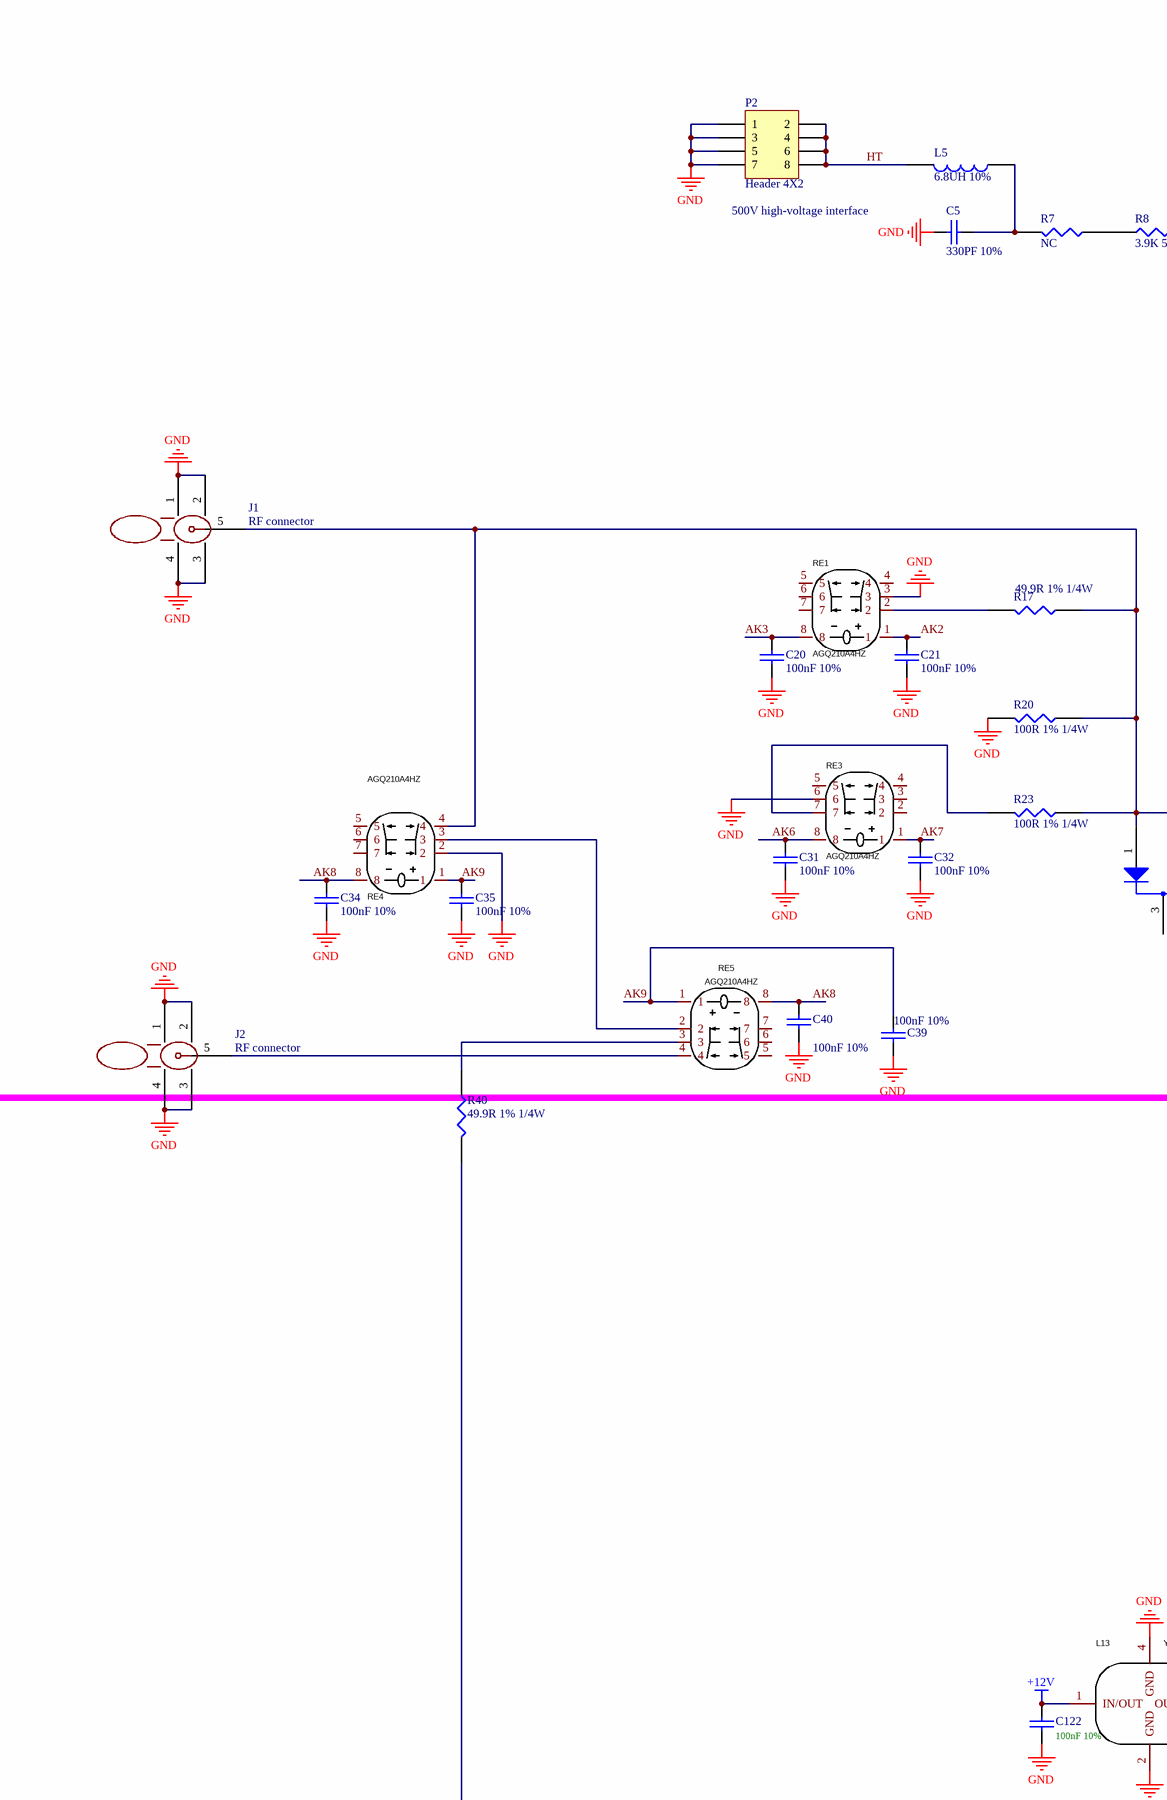
[diagram p0: PCBE109560-11.SchDoc, top left]
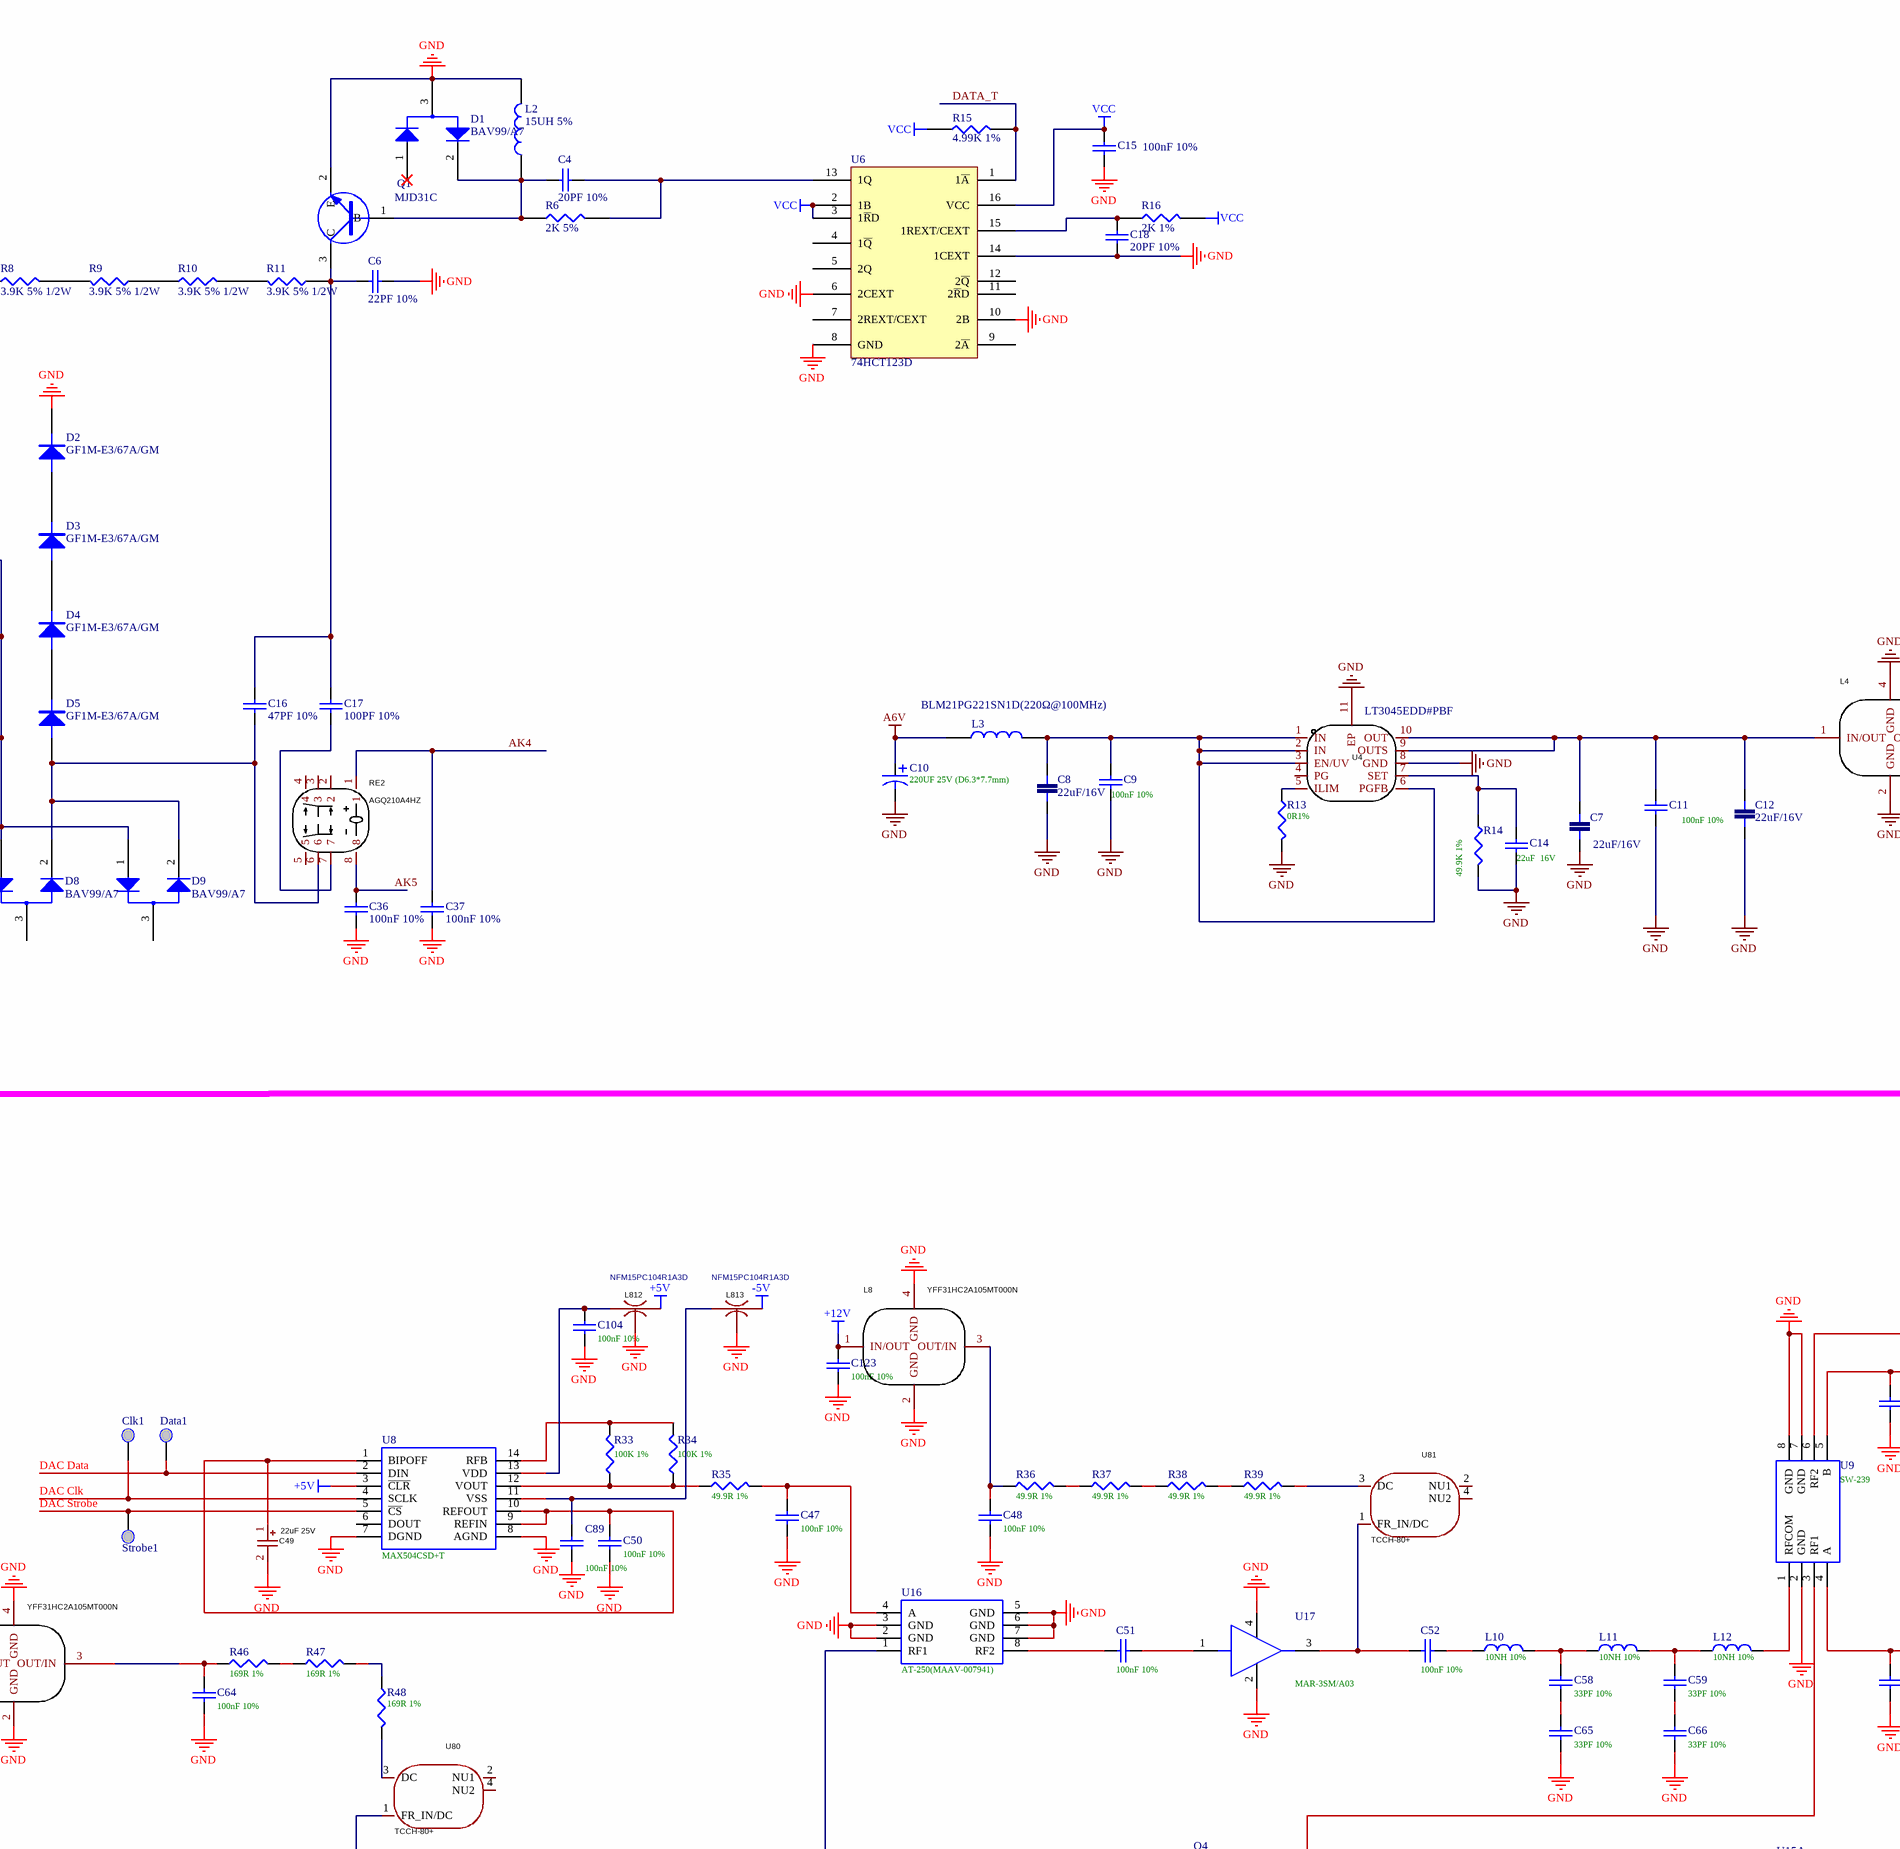
[diagram p1: PCBE109560-11.SchDoc, top middle]
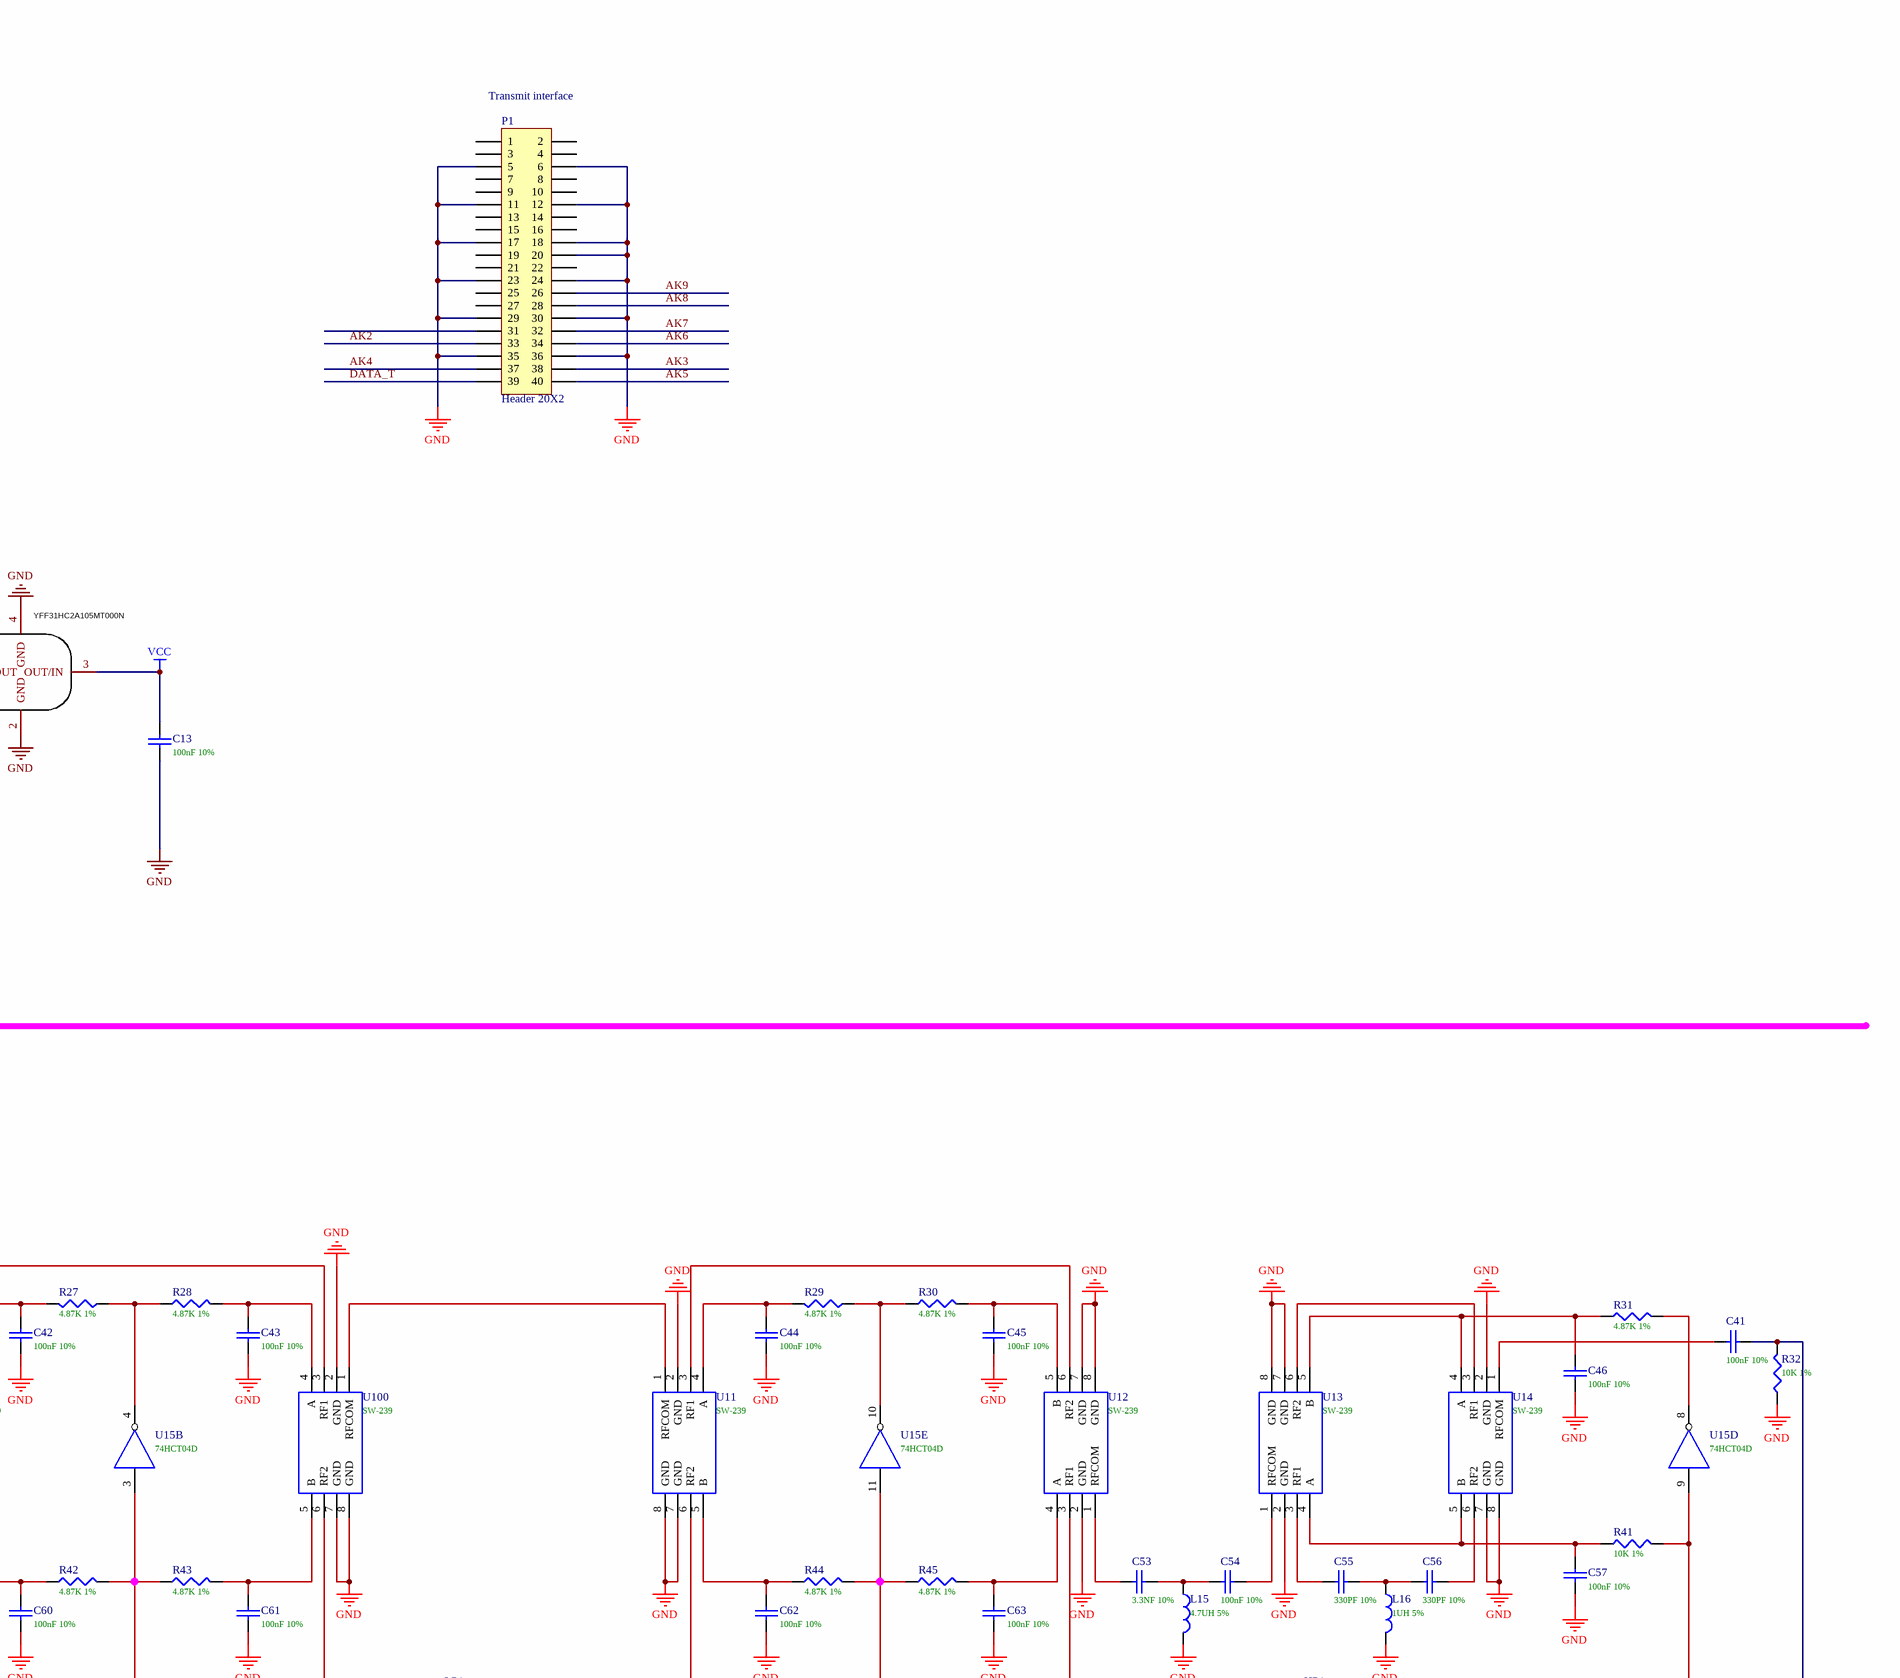
[diagram p2: PCBE109560-11.SchDoc, top right]
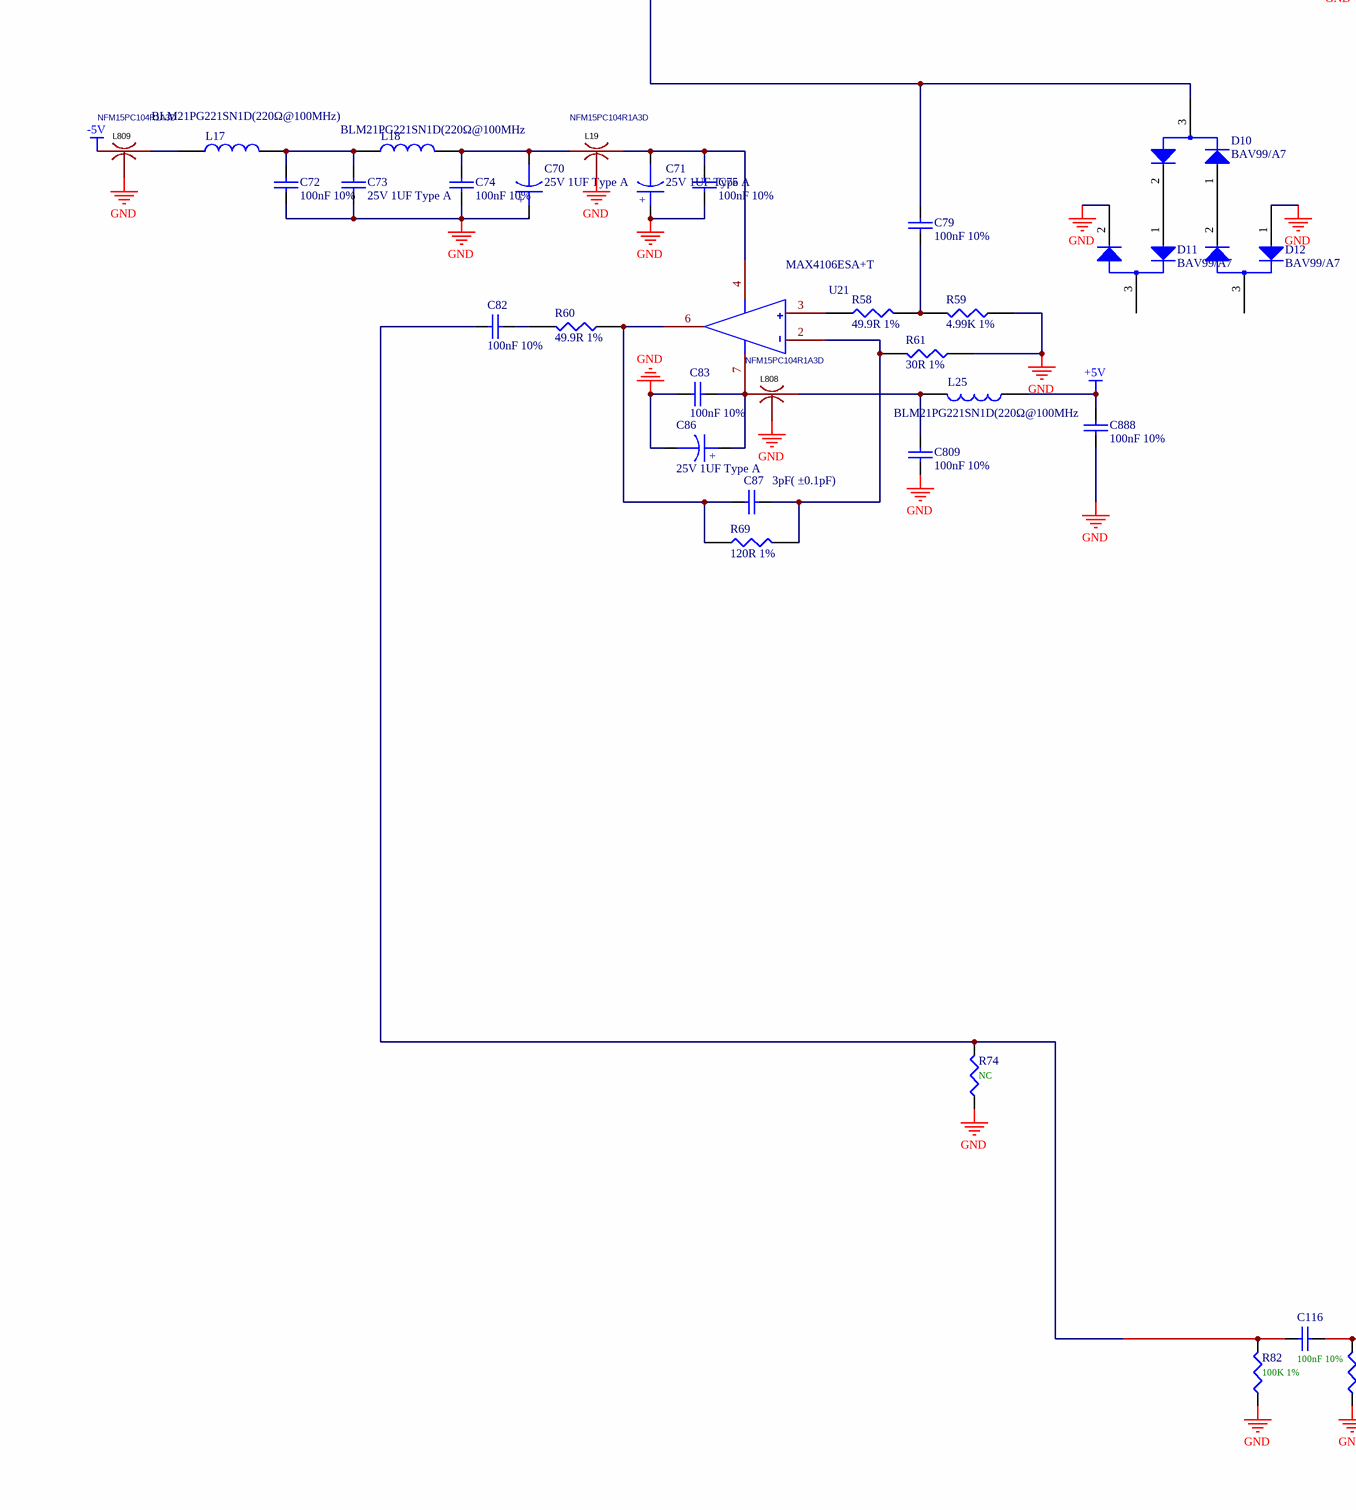
[diagram p3: PCBE109560-11.SchDoc, bottom left]
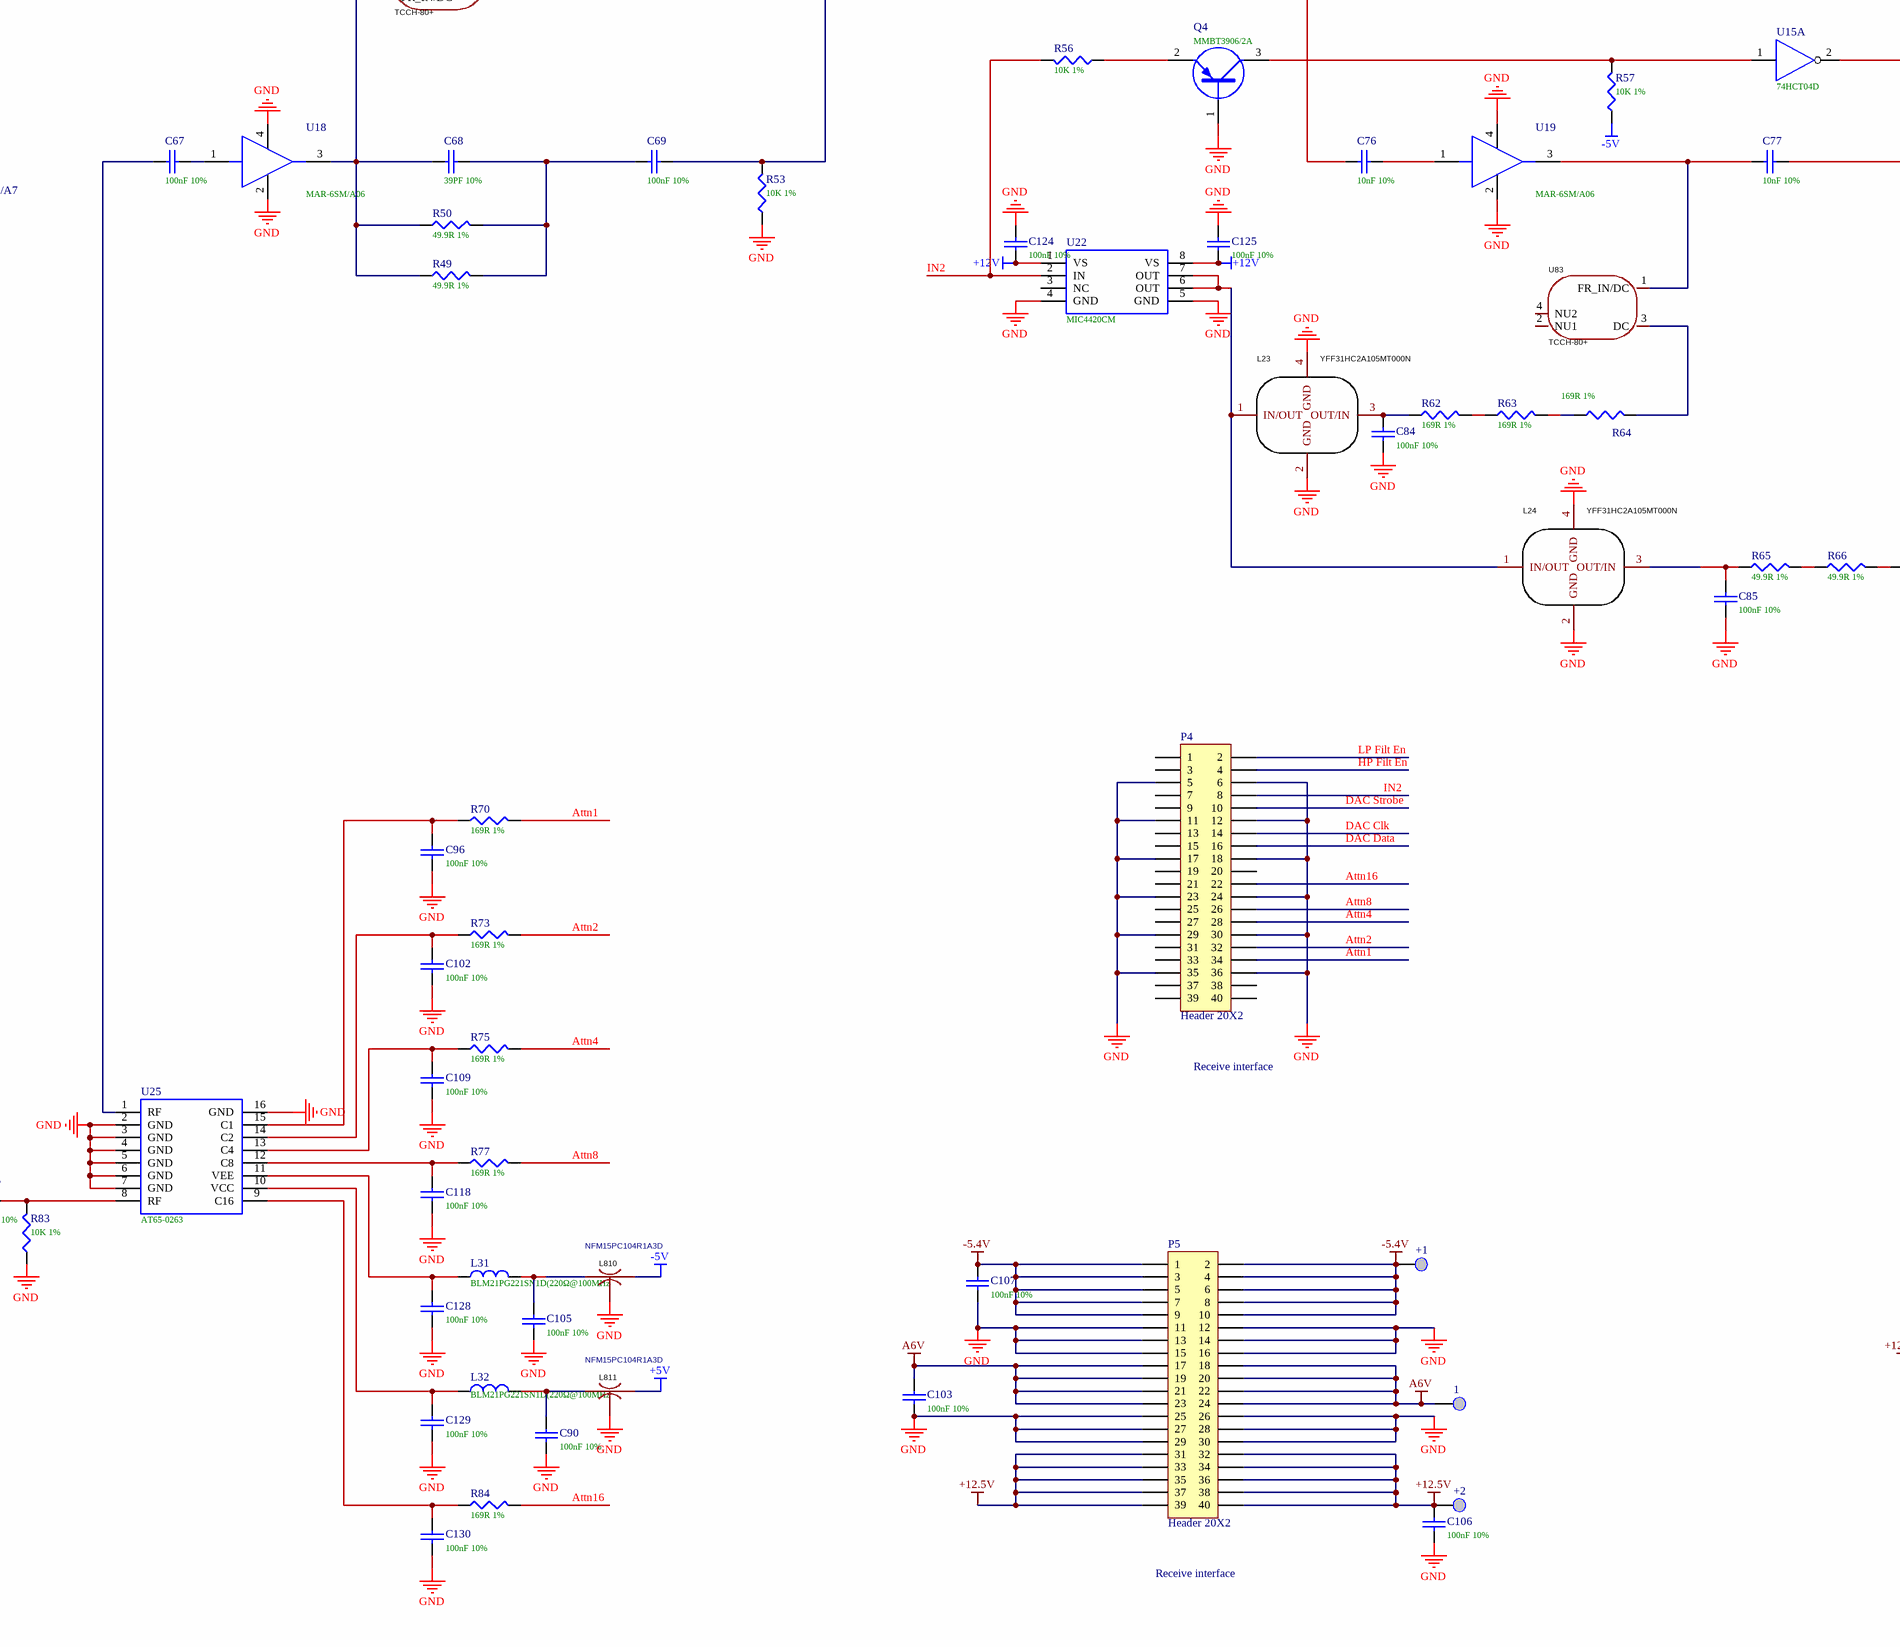
[diagram p4: PCBE109560-11.SchDoc, bottom middle]
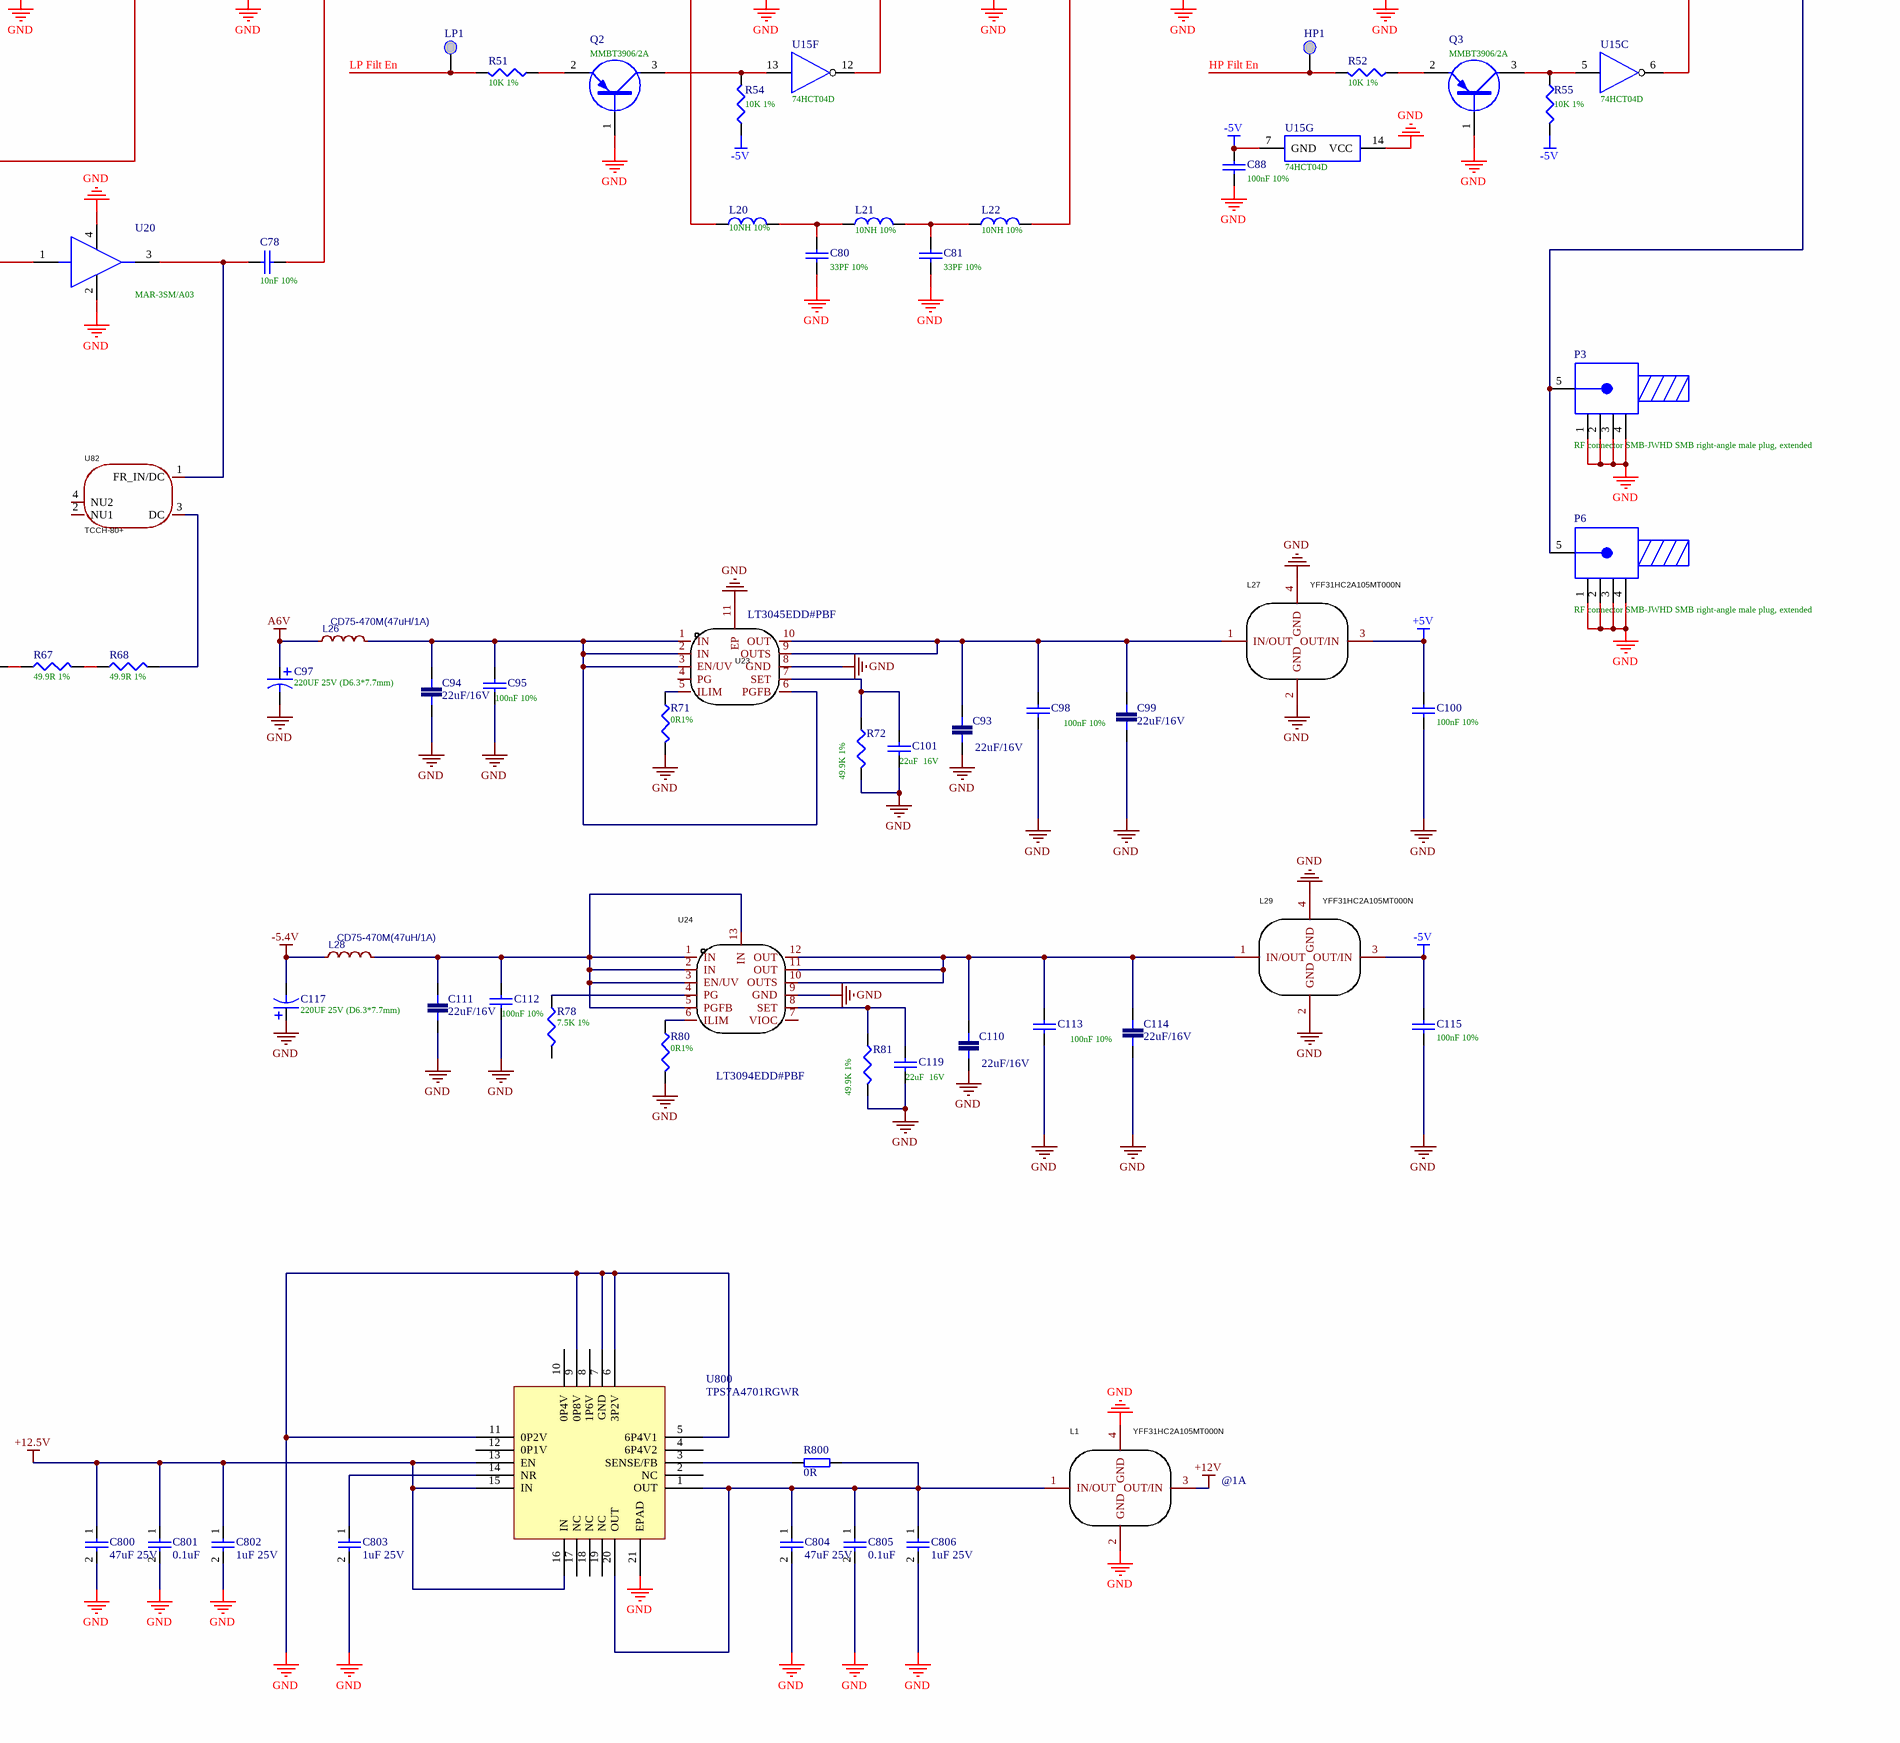
[diagram p5: PCBE109560-11.SchDoc, bottom right]
# Altium schematic sheet PCBE109560-11.SchDoc (part 1 of 2)
size E; SheetNumber: 0; SheetTotal: 0